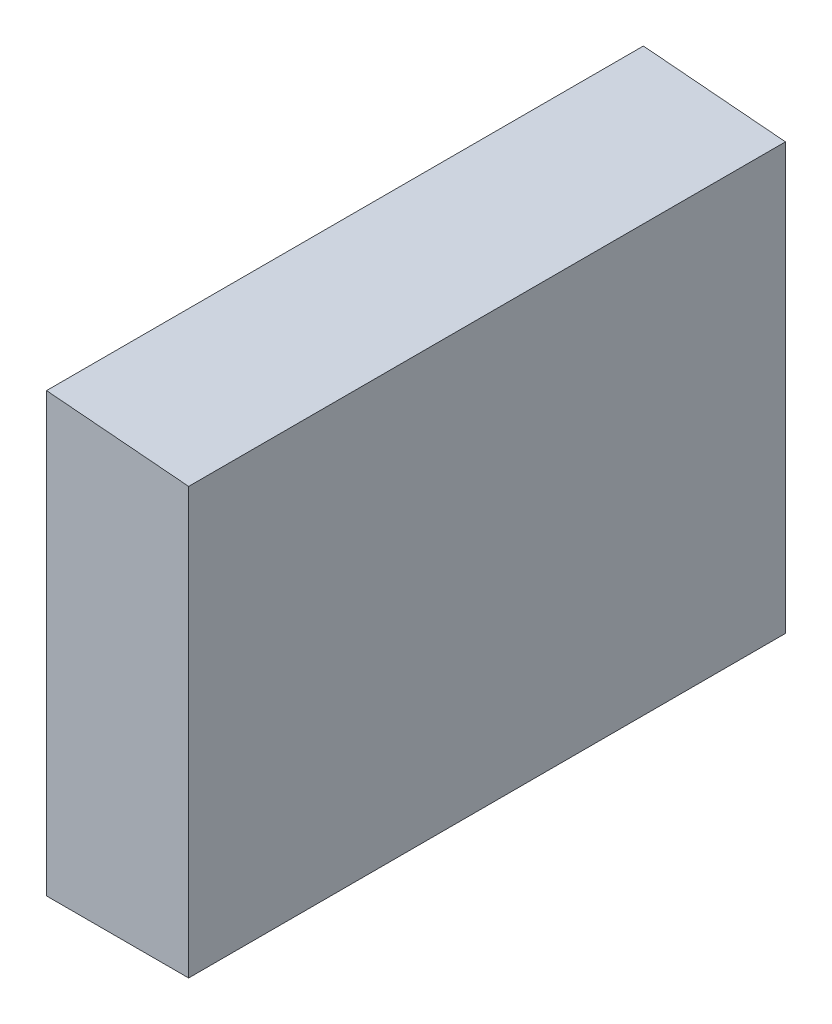
from build123d import *

# Parameters (mm, degrees)
BOSS_EXTRUDE1_DEPTH = 42


with BuildPart() as part:
    # Sketch1 → Boss-Extrude1 (new body)
    with BuildSketch(Plane.XY):
        Polygon((0, 30.8), (10, 29.960276538), (10, 0), (0, 0), align=None)
    extrude(amount=BOSS_EXTRUDE1_DEPTH)


solid = part.part
